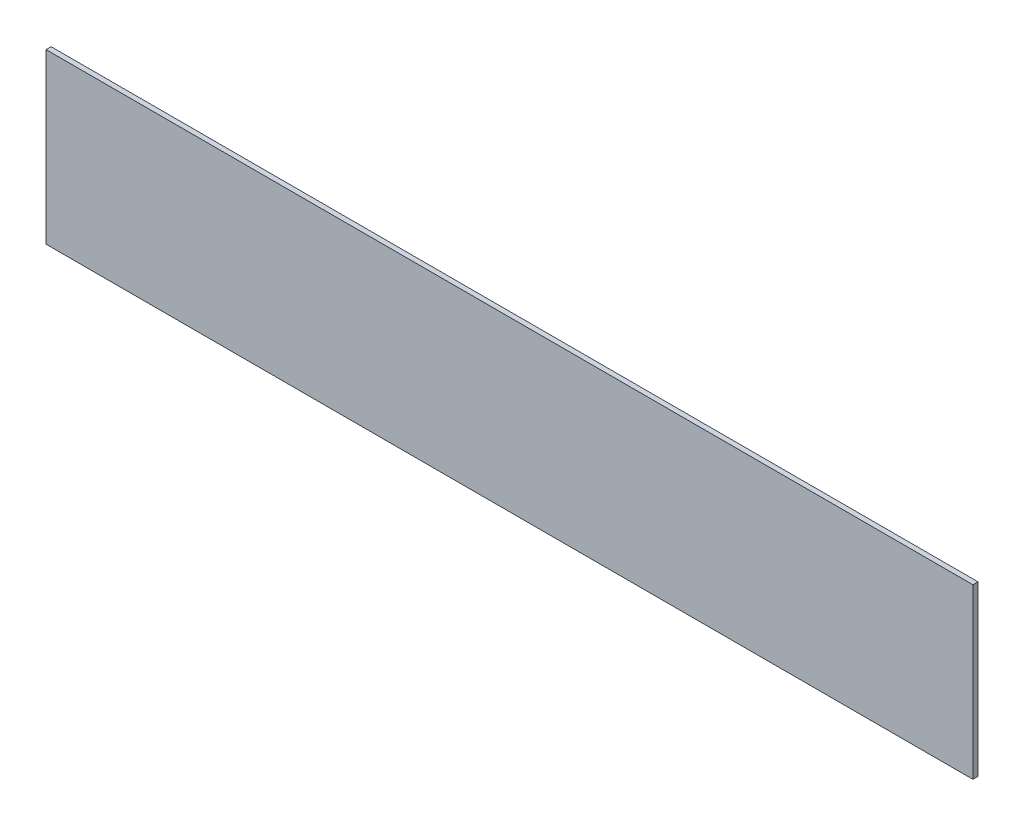
SolidWorks part; units mm, degrees
ref_plane "前视基准面" through (0, 0, 0) normal (0, 0, 1) x (1, 0, 0)
ref_plane "上视基准面" through (0, 0, 0) normal (0, 1, 0) x (1, 0, 0)
ref_plane "右视基准面" through (0, 0, 0) normal (1, 0, 0) x (0, 0, -1)
other "Configuration Table"
sketch "草图1" plane through (0, 0, 0) normal (0, 0, 1) x (1, 0, 0)
  line L1 (275, -50) -> (-275, -50)
  line L2 (275, -50) -> (275, 50)
  line L3 (275, 50) -> (-275, 50)
  line L4 (-275, -50) -> (-275, 50)
  line L5 (275, -50) -> (-275, 50) construction
  line L6 (275, 50) -> (-275, -50) construction
  point P0 (0, 0)
  dimension "D1" = 100
  dimension "D2" = 550
extrude "凸台-拉伸1" add sketch "草图1" along normal blind 3
